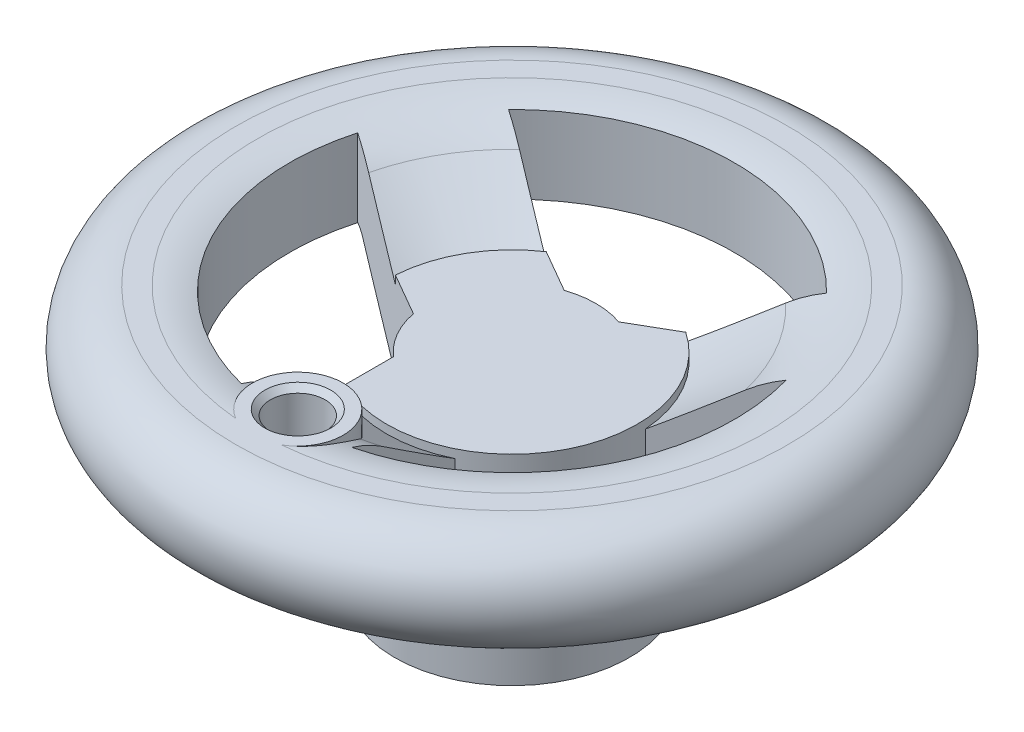
from build123d import *

# Parameters (mm, degrees)
CUT_EXTRUDE1_DEPTH = 32
SKETCH5_W          = 5.5
SKETCH5_H          = 13
CIRPATTERN1_COUNT  = 3


with BuildPart() as part:
    # Sketch1 → Revolve1 (revolve)
    with BuildSketch(Plane.XY, mode=Mode.PRIVATE) as revolve1_sk:
        with BuildLine():
            Line((0, 20), (5, 20))
            Line((5, 20), (5, 16.939442451))
            Line((5, 16.939442451), (23.498601429, 29.700772791))
            ThreePointArc((23.498601429, 29.700772791), (27.014696752, 31.411890394), (30.880570115, 32))
            Line((30.880570115, 32), (33.5, 32))
            ThreePointArc((33.5, 32), (39.438608051, 22.857475748), (28.671410524, 21.148595207))
            ThreePointArc((28.671410524, 21.148595207), (27.10540909, 21.957966627), (25.394651363, 21.5328189))
            Line((25.394651363, 21.5328189), (5, 7.463491323))
            Line((5, 7.463491323), (5, 2))
            Line((5, 2), (0, 2))
            Line((0, 2), (0, 20))
        make_face()
    revolve(revolve1_sk.sketch.rotate(Axis((0, 0, 0), (0, 1, 0)), 270), axis=Axis((0, 0, 0), (0, 1, 0)))

    # Sketch2 → Cut-Extrude1 (cut)
    with BuildSketch(Plane(origin=(0, 0, 0), x_dir=(1, 0, 0), z_dir=(0, 1, 0))):
        with BuildLine():
            Line((26.001324465, 7.275378072), (10.010517998, -1.956918346))
            ThreePointArc((10.010517998, -1.956918346), (8.833459119, -5.1), (6.7, -7.690903718))
            Line((6.7, -7.690903718), (6.7, -26.155496554))
            ThreePointArc((6.7, -26.155496554), (23.382685902, -13.5), (26.001324465, 7.275378072))
        make_face()
    cut_extrude1 = extrude(amount=CUT_EXTRUDE1_DEPTH, mode=Mode.SUBTRACT)

    # Sketch4 → Revolve2 (revolve)
    with BuildSketch(Plane.XY, mode=Mode.PRIVATE) as revolve2_sk:
        Polygon((0, 25), (15.2, 25), (15.2, 8.9), (14.25, 8.9), (14.25, 0), (0, 0), align=None)
    revolve(revolve2_sk.sketch.rotate(Axis((0, 0, 0), (0, 1, 0)), 270), axis=Axis((0, 0, 0), (0, 1, 0)))

    # Sketch5 → Revolve3 (revolve)
    with BuildSketch(Plane(origin=(0, 0, 0), x_dir=(0, 0, -1), z_dir=(1, 0, 0))):
        with Locations((-23.25, 25.5)):
            Rectangle(SKETCH5_W, SKETCH5_H)
    revolve(axis=Axis((0, 19, 26), (0, 1, 0)))

    # Sketch6 → Cut-Revolve1 (revolve, cut)
    with BuildSketch(Plane(origin=(0, 0, 0), x_dir=(0, 0, -1), z_dir=(1, 0, 0)), mode=Mode.PRIVATE) as cut_revolve1_sk:
        Polygon((-26, 32), (-22, 32), (-22.6765, 31.3235), (-22.6765, 19.6765), (-22, 19), (-26, 19), align=None)
    revolve(cut_revolve1_sk.sketch.rotate(Axis((0, 19, 26), (0, 1, 0)), 180), axis=Axis((0, 19, 26), (0, 1, 0)), mode=Mode.SUBTRACT)

    # Sketch7 → Cut-Revolve2 (revolve, cut)
    with BuildSketch(Plane.XY, mode=Mode.PRIVATE) as cut_revolve2_sk:
        Polygon((0, 11.732050808), (3, 10), (3, 0), (0, 0), align=None)
    revolve(cut_revolve2_sk.sketch.rotate(Axis((0, 0, 0), (0, 1, 0)), 270), axis=Axis((0, 0, 0), (0, 1, 0)), mode=Mode.SUBTRACT)

    # CirPattern1: Cut-Extrude1 ×3 about axis
    cirpattern1_axis = Axis((0, 0, 0), (0, 1, 0))
    for i in range(1, CIRPATTERN1_COUNT):
        add(cut_extrude1.rotate(cirpattern1_axis, i * 360 / CIRPATTERN1_COUNT), mode=Mode.SUBTRACT)


solid = part.part
